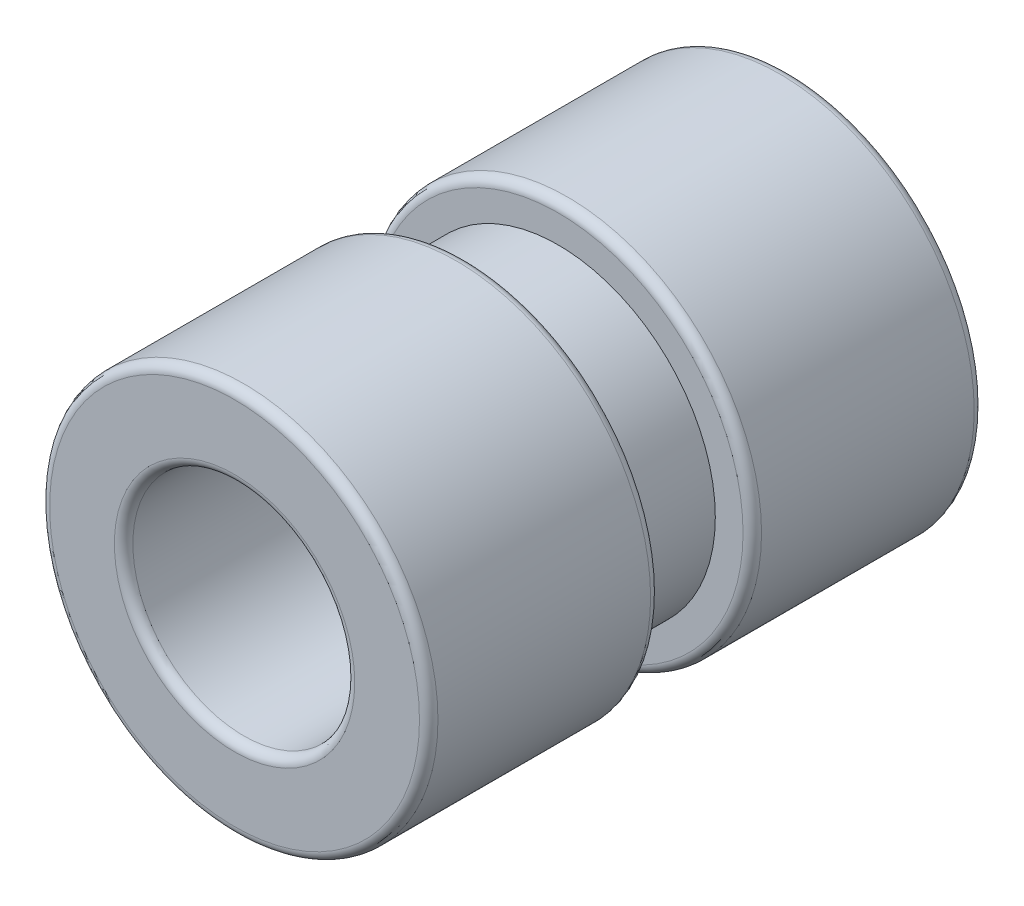
SolidWorks part; units mm, degrees
material "Copper"
ref_plane "Front Plane" through (0, 0, 0) normal (0, 0, 1) x (1, 0, 0)
ref_plane "Top Plane" through (0, 0, 0) normal (0, 1, 0) x (1, 0, 0)
ref_plane "Right Plane" through (0, 0, 0) normal (1, 0, 0) x (0, 0, -1)
sketch "Sketch1" plane through (0, 0, 0) normal (0, 0, 1) x (1, 0, 0)
  line L0 (0, 0) -> (0, 51.8131) construction
  circle A0 centre (0, 0) radius 10.5
  circle A1 centre (0, 0) radius 6
  dimension "D1" = 12
  dimension "D2" = 21
extrude "Boss-Extrude1" add sketch "Sketch1" along normal mid plane 30
sketch "Sketch2" plane through (0, 0, 0) normal (0, 0, 1) x (1, 0, 0)
  circle A0 centre (0, 0) radius 8.5
  circle A1 centre (0, 0) radius 14.1133
  dimension "D1" = 17
extrude "Cut-Extrude1" cut sketch "Sketch2" against normal mid plane 5
fillet "Fillet1" radius 0.5 6 edges at (6, 0, -15) (6, 0, 15) (10.5, 0, -15) (10.5, 0, 15) (10.5, 0, 2.5) (10.5, 0, -2.5)
